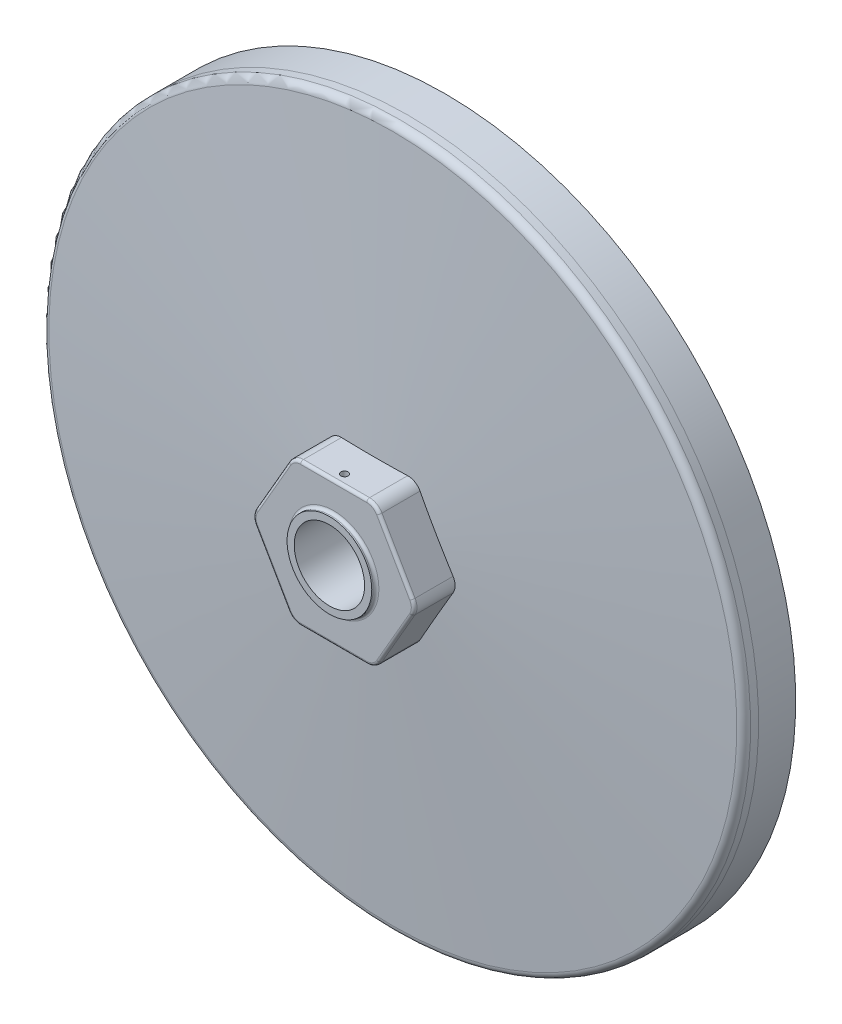
from build123d import *

# Parameters (mm, degrees)
SKETCH1_R           = 2.458734123
BOSS_EXTRUDE_DEPTH  = 3.2
CUT_EXTRUDE1_DEPTH  = 3
FILLET1_R           = 0.5
FILLET2_R           = 1
SKETCH7_R           = 2.958734123
SKETCH7_R_2         = 2.458734123
EXTRUDE_THIN1_DEPTH = 0.3
FILLET3_R           = 0.2
SKETCH8_R           = 0.25
CUT_EXTRUDE2_DEPTH  = 4.3
CUT_EXTRUDE3_START  = -14.3
SKETCH9_R           = 2.458734123
CUT_EXTRUDE3_DEPTH  = 14.3
SCALE1_SCALE        = 2.7
SKETCH10_R          = 66.157826775
SKETCH10_R_2        = 63.157826775
EXTRUDE_THIN2_DEPTH = 7


with BuildPart() as part:
    # Sketch1 → Boss-Extrude (new, symmetric)
    with BuildSketch(Plane.XY):
        Polygon((2.8875, 5.001296707), (-2.8875, 5.001296707), (-5.775, 0), (-2.8875, -5.001296707), (2.8875, -5.001296707), (5.775, 0), align=None)
        Circle(SKETCH1_R, mode=Mode.SUBTRACT)
    extrude(amount=BOSS_EXTRUDE_DEPTH, both=True)

    # Sketch5 → Revolve1 (revolve)
    with BuildSketch(Plane(origin=(0, 0, 0), x_dir=(0, 0, -1), z_dir=(1, 0, 0))):
        Polygon((2.275194756, 0), (3.964011499, 24.502523336), (4.988616082, 24.502523336), (4.988616082, 0), align=None)
    revolve(axis=Axis((0, 0, -2.275194756), (0, 0, -1)))

    # Sketch6 → Cut-Extrude1 (cut)
    with BuildSketch(Plane.XY.offset(3.2)):
        Polygon((5.775, 0), (2.8875, 5.001296707), (-2.8875, 5.001296707), (-5.775, 0), (-2.8875, -5.001296707), (2.8875, -5.001296707), align=None)
    extrude(amount=-CUT_EXTRUDE1_DEPTH, mode=Mode.SUBTRACT)

    # Fillet1
    fillet1_edges = [part.edges().sort_by_distance(p)[0] for p in [
        (0, -24.502523336, -3.964011499),
    ]]
    fillet(fillet1_edges, radius=FILLET1_R)

    # Fillet2
    fillet2_edges = [part.edges().sort_by_distance(p)[0] for p in [
        (-2.8875, -5.001296707, -1.236615997),
        (2.8875, -5.001296707, -1.236615997),
        (5.775, 0, -1.236615997),
        (-2.8875, 5.001296707, -1.236615997),
        (-5.775, 0, -1.236615997),
        (2.8875, 5.001296707, -1.236615997),
    ]]
    fillet(fillet2_edges, radius=FILLET2_R)

    # Sketch7 → Extrude-Thin1 (add)
    with BuildSketch(Plane.XY.offset(0.2)):
        Circle(SKETCH7_R)
        Circle(SKETCH7_R_2, mode=Mode.SUBTRACT)
    extrude(amount=EXTRUDE_THIN1_DEPTH)

    # Fillet3
    fillet3_edges = [part.edges().sort_by_distance(p)[0] for p in [
        (-2.958734123, 0, 0.2),
        (0, -5.001296707, 0.2),
        (-4.33125, -2.500648353, 0.2),
        (4.33125, -2.500648353, 0.2),
        (4.33125, 2.500648353, 0.2),
        (0, 5.001296707, 0.2),
        (-4.33125, 2.500648353, 0.2),
        (2.810149731, 4.867322111, 0.2),
        (-5.620299462, 0, 0.2),
        (-2.810149731, 4.867322111, 0.2),
        (5.620299462, 0, 0.2),
        (2.810149731, -4.867322111, 0.2),
        (-2.810149731, -4.867322111, 0.2),
    ]]
    fillet(fillet3_edges, radius=FILLET3_R)

    # Sketch8 → Cut-Extrude2 (cut)
    with BuildSketch(Plane(origin=(0, 5.001296707, 0), x_dir=(1, 0, 0), z_dir=(0, 1, 0))):
        with Locations(Location((0, 0.558219382, 0), (0, 0, 180))):
            Circle(SKETCH8_R)
    extrude(amount=-CUT_EXTRUDE2_DEPTH, mode=Mode.SUBTRACT)

    # Sketch9 → Cut-Extrude3 (cut)
    with BuildSketch(Plane.XY.offset(CUT_EXTRUDE3_START)):
        with Locations(Location((0, 0, 0), (0, 0, 270))):
            Circle(SKETCH9_R)
    extrude(amount=CUT_EXTRUDE3_DEPTH, mode=Mode.SUBTRACT)


with BuildPart() as part_1:
    # Scale1: scaled about (1.23e-07, -0.000596522, -3.973390116)
    add(part.part.scale(SCALE1_SCALE).moved(Location((-2.09e-07, 0.001014087, 6.754763197))))

    # Sketch10 → Extrude-Thin2 (add)
    with BuildSketch(Plane(origin=(0, 0, -6.714499546), x_dir=(-1, 0, 0), z_dir=(0, 0, -1))):
        Circle(SKETCH10_R)
        Circle(SKETCH10_R_2, mode=Mode.SUBTRACT)
    extrude(amount=EXTRUDE_THIN2_DEPTH)


solid = part_1.part
